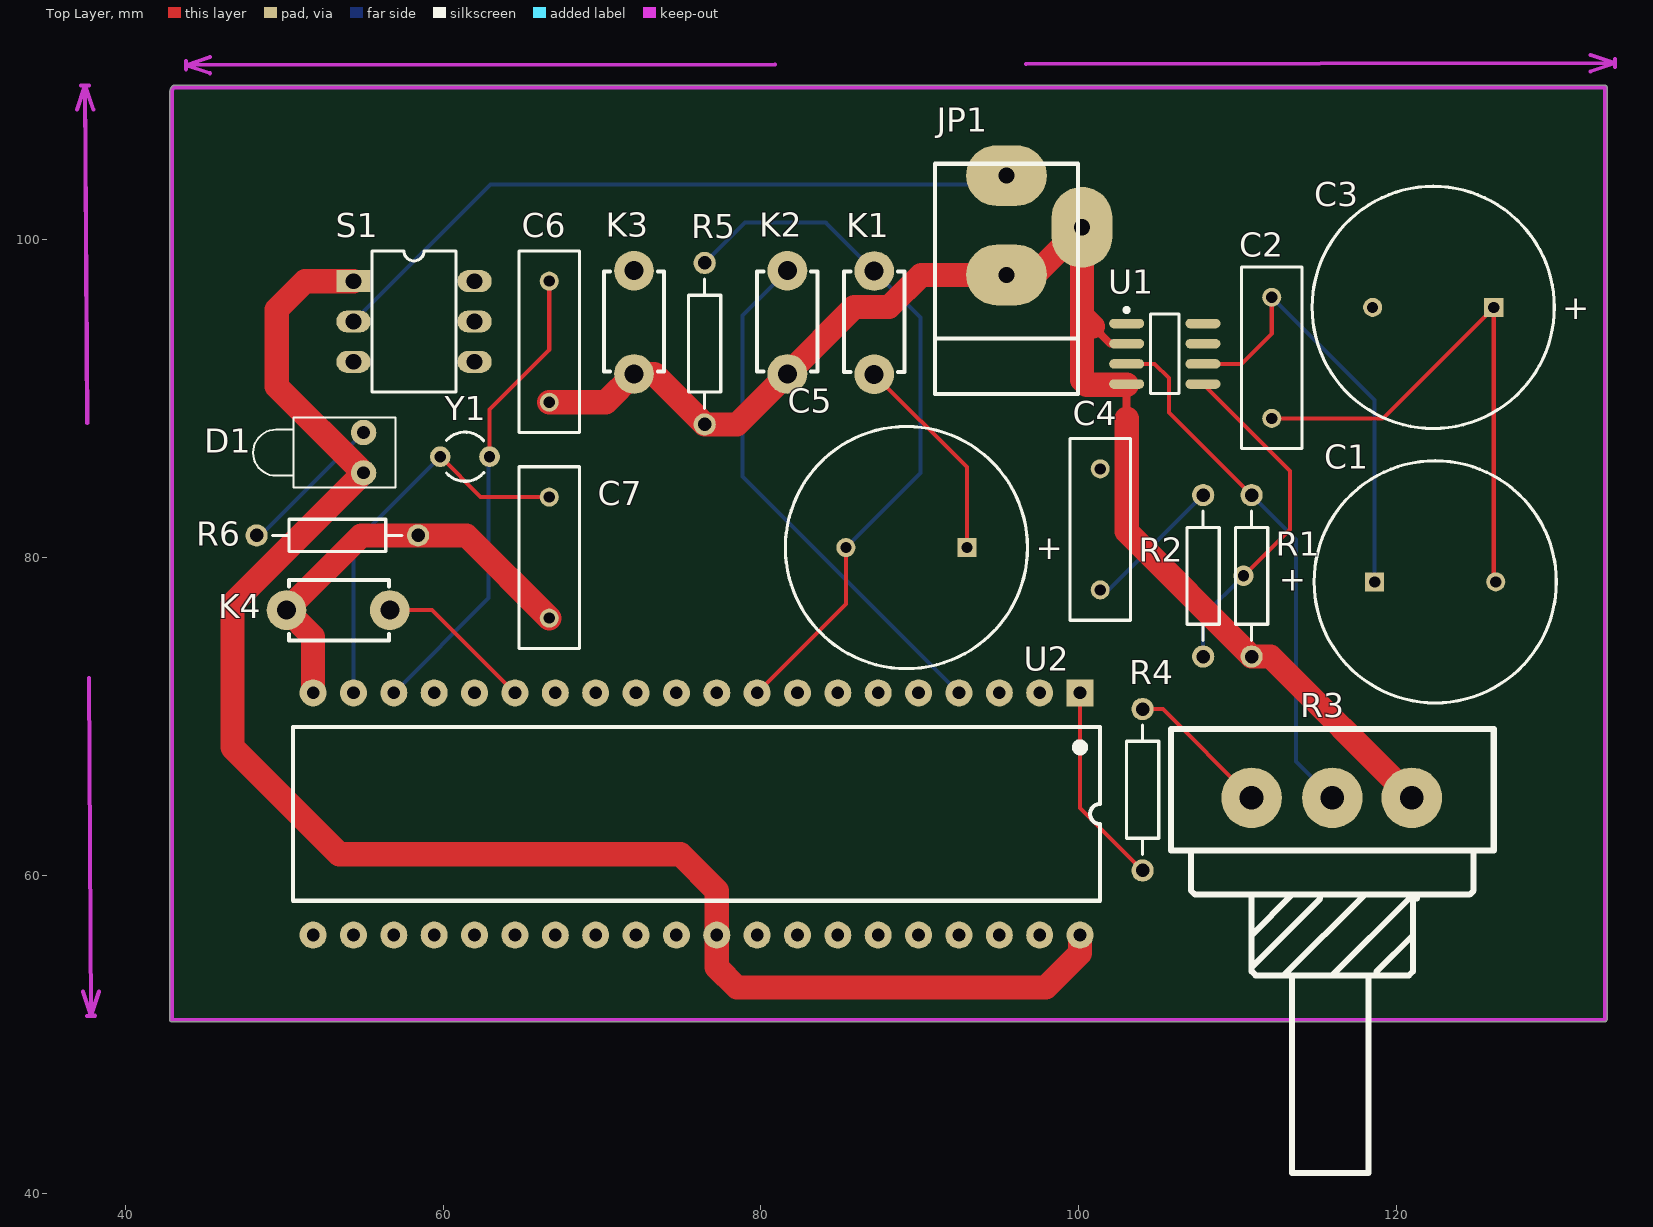
[diagram p0: Top Layer view]
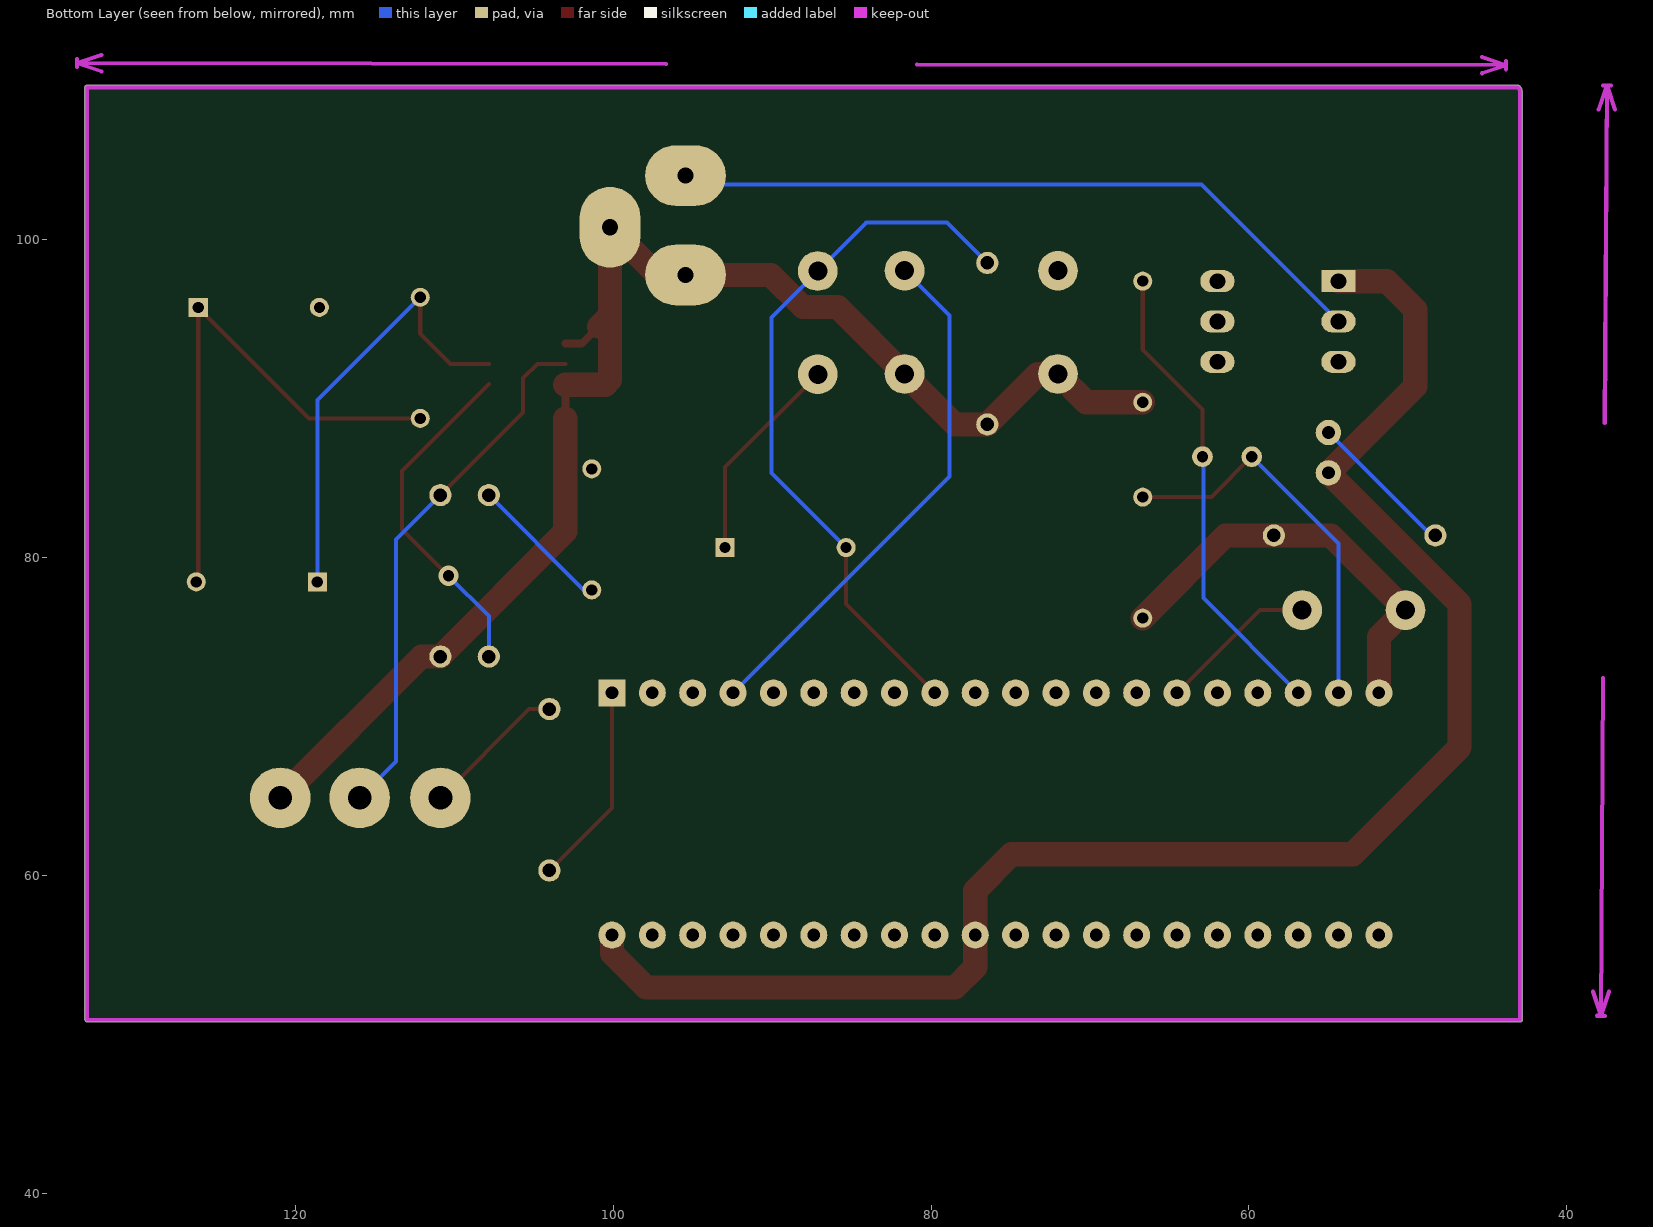
[diagram p1: Bottom Layer view, seen from below]
# Altium PCB MISC82808.PcbDoc
Units mm, origin at the board's own origin, x right, y up, seen from the top; angles counter-clockwise.
Board outline 90.45 x 58.93 mm, 2 copper layers (Top Layer, Bottom Layer); 23 components, 20 nets, 96 pads, 1 vias.
Unrouted connection lines stored in the file: 2.

## Layer stack, top to bottom (the 12.6 mil dielectric is the usual default, probably not edited)
Top Solder: solder mask 0.0102, Solder Resist, Dk 3.5
Top Layer: signal copper 0.0356
Dielectric 1: dielectric 0.32, FR-4, Dk 4.8
Bottom Layer: signal copper 0.0356
Bottom Solder: solder mask 0.0102, Solder Resist, Dk 3.5

## Board outline
42.926,50.8 cw(c42.926,50.927) 42.799,50.927 42.799,109.294 cw(c43.36,109.294) 42.963,109.691 cw(c43.053,109.601) 43.053,109.728 133.118,109.728 cw(c133.118,109.601) 133.245,109.601 133.245,50.98 cw(c133.043,50.98) 133.186,50.837 cw(c133.096,50.927) 133.096,50.8

## Design rules (kind name [scope] priority, off if disabled: settings)
Clearance [All] p1: gap=0.254
PolygonConnect [All] p1: connectstyle=Relief reliefconductorwidth=0.254 reliefentries=4 polygonreliefangle="90 Angle" airgapwidth=0.254
RoutingVias [All] p1: holewidth=0.711 width=1.27 viastyle="Through Hole" minholewidth=0.711 minwidth=1.27 maxholewidth=0.711 maxwidth=1.27
SolderMaskExpansion [All] p1: expansion=0.102
Width [All] p1: maxlimit=254 minlimit=0.254 preferedwidth=0.254 toplayer_maxwidth=25.4 minimp=50.000000 maximp=50.000000 favimp=50.000000
30 further rules are at their usual default settings.

## Classes and differential pairs
component class ZBW172: B1 C1 C3 C4 C5 C6 C7 D1 JP1 K1 K2 K3 K4 R3 R4 R5 R6 S1 U1 U2 Y1

## Components (designator, comment, footprint, x,y, rotation, side; value= is the part's Value field where it differs from the comment)
C1 "Cap Pol1" RB7.6-15 122.428,78.486 r180 top
C2 "Cap" RAD-0.3 112.141,92.583 r270 top
C3 "Cap Pol1" RB7.6-15 122.301,95.758 r0 top
C4 "Cap" RAD-0.3 101.346,81.788 r90 top
C5 "Cap Pol1" RB7.6-15 89.154,80.645 r0 top
C6 "Cap" RAD-0.3 66.675,93.599 r90 top
C7 "Cap" RAD-0.3 66.675,80.01 r90 top
D1 "LED1" LED-1 54.991,86.614 r180 top
JP1 "DC 5V" "DC POWER JACK1" 99.949,90.297 r90 top
K1 "KEY" DIP-3X6X4.3 87.122,91.544 r90 top
K2 "KEY" DIP-3X6X4.3 81.661,91.567 r90 top
K3 "KEY" DIP-3X6X4.3 72.009,91.567 r90 top
K4 "KEY" DIP-3X6X4.3 50.142,76.708 r0 top
R1 "Res2" AXIAL-0.4 110.871,78.867 r90 top
R2 "Res2" AXIAL-0.4 107.823,78.867 r90 top
R3 "Potentiometer" 滑动变阻器 115.951,55.245 r0 top
R4 "Res2" AXIAL-0.4 104.013,65.405 r90 top
R5 "Res2" AXIAL-0.4 76.454,93.472 r90 top
R6 "Res2" AXIAL-0.4 53.34,81.407 r0 top
S1 "SW3-DIP6" DIP-Switch3 54.356,97.409 r0 top
U1 "LM386" M08A_N 105.41,92.837 r0 top
U2 "STC89C51" DIP40 75.946,63.881 r270 top
Y1 "XTAL" R38 61.367,86.36 r90 top

## Footprints (in the part's own frame and the unit in brackets; to place one, negate y for a bottom-side part, rotate by r counter-clockwise, add the part's x,y. Pads: shape width x height; smd on the part's side, far side on the other; paste and mask are expansions set on the pad)
AXIAL-0.4 [mm] "Axial Device, Thru-Hole; 2 Leads; 0.4 in Pin Spacing"
  round 1.4 hole 0.85: 1(-5.08,0) 2(5.08,0)
  silkscreen extent -4.06,-1.02 4.06,1.02
"DC POWER JACK1" [mm] "ª½¬y¹q·½´¡®y"
  oval 3.81x5.08 hole 1.016: 1(13.75,4.5) 2(7.5,4.5)
  oval 5.08x3.81 hole 1.016: 3(10.5,-0.25)
  silkscreen extent 0,0 14.5,9
DIP40 [mm]
  rect 1.7x1.7 hole 0.8: 1(-7.62,24.13)
  round 1.7 hole 0.8: 2(-7.62,21.59) 3(-7.62,19.05) 4(-7.62,16.51) 5(-7.62,13.97) 6(-7.62,11.43) 7(-7.62,8.89) 8(-7.62,6.35) 9(-7.62,3.81) 10(-7.62,1.27) 11(-7.62,-1.27) 12(-7.62,-3.81) 13(-7.62,-6.35) 14(-7.62,-8.89) 15(-7.62,-11.43) 16(-7.62,-13.97) 17(-7.62,-16.51) 18(-7.62,-19.05) 19(-7.62,-21.59) 20(-7.62,-24.13) 21(7.62,-24.13) 22(7.62,-21.59) 23(7.62,-19.05) 24(7.62,-16.51) 25(7.62,-13.97) 26(7.62,-11.43) 27(7.62,-8.89) 28(7.62,-6.35) 29(7.62,-3.81) 30(7.62,-1.27) 31(7.62,1.27) 32(7.62,3.81) 33(7.62,6.35) 34(7.62,8.89) 35(7.62,11.43) 36(7.62,13.97) 37(7.62,16.51) 38(7.62,19.05) 39(7.62,21.59) 40(7.62,24.13)
  silkscreen extent -5.46,-25.4 5.46,25.4, body extent -7.91,-26.19 7.65,26.16, height 4.7
DIP-3X6X4.3 [mm]
  round 2.5 hole 1.2: 1(0,0) 3(6.5,0)
  silkscreen extent 0.16,-1.9 6.46,1.9, body extent -0.64,-1.75 7.19,1.75, height 4.31
DIP-Switch3 [mil]
  rect 85x55 hole 39 paste+0 mask+4: 1(0,0)
  oval 85x55 hole 39 paste+0 mask+4: 2(0,-100) 3(0,-200) 4(300,-200) 5(300,-100) 6(300,0)
  silkscreen extent 46,-275 254,75, body extent -55,-271 359,67, height 153
LED-1 [mm] "LED; 2 Leads"
  round 1.6 hole 0.8: 1(0,1.27) 2(0,-1.27)
  silkscreen extent -2,-2.2 6.95,2.2
M08A_N [mm] "SOIC, 8-Leads, Body 4.9x3.9mm, Pitch 1.27mm, IPC Medium Density"
  oval 2.2x0.6 smd: 1(-2.4,1.905) 2(-2.4,0.635) 3(-2.4,-0.635) 4(-2.4,-1.905) 5(2.4,-1.905) 6(2.4,-0.635) 7(2.4,0.635) 8(2.4,1.905)
  silkscreen extent -2.52,-2.5 0.9,2.88, body extent -2,-2.5 2,2.5, height 1.75
R38 [mm] "Crystal, Thru-Hole; 2 Leads; Body 3.1 x 8.2 mm (Dia.xH)"
  round 1.3 hole 0.7: 1(0,1.55) 2(0,-1.55)
  silkscreen extent -1.55,-1.19 1.55,1.17
RAD-0.3 [mm] "Radial Cap, Thru-Hole; 2 Leads; 0.3 in Pin Spacing"
  round 1.2 hole 0.7: 1(-3.81,0) 2(3.81,0)
  silkscreen extent -5.71,-1.91 5.71,1.91
RB7.6-15 [mm] "Polarized Capacitor (Radial); 2 Leads"
  rect 1.2x1.2 hole 0.7: 1(3.81,0)
  round 1.2 hole 0.7: 2(-3.81,0)
  silkscreen extent -7.62,-7.62 7.62,7.62
滑动变阻器 [mil]
  round 150 hole 59.06 paste+0 mask+4: 1(-200,380) 3(196.85,380)
  round 150 hole 59.05 paste+4 mask+4: 2(0,380)
  silkscreen extent -400,-550 400,550

## Part data
C1 C3 C5: "Polarized Capacitor (Radial)"
C2 C4 C6 C7: "Capacitor"
D1: "Typical RED GaAs LED"
JP1: library part "DC POWER JACK1", "DC power jack"
R1 R2 R4 R5 R6: "Resistor"
R3: library part 滑动变阻器
U1: library part LM386M-1, "Low Voltage Audio Power Amplifier, 8-pin Narrow SOIC"
Y1: "Crystal Oscillator"

## Via types
v1: diameter 1.27, hole 0.711, Top Layer to Bottom Layer, 1 vias

## Nets (pads, with @x,y where several pads share a name; then routed paths per layer and width w, separated by ;. In a path a pad name is that pad's centre, name@x,y a point inside that pad or via, vN(x,y) a via of type N, cw(c..) or ccw(c..) an arc to the next point about the centre after c; other vN are vias at no path point)
GND: C6.1 C7.1 JP1.2 JP1.3 K2.1 K3.1 K4.1 R1.1 R3.3 R5.1 R6.2 U1.2 U1.4 U2.20 | length 117.5
  Top Layer w0.508: 100.894,94.559 101.981,93.472 U1.2 ; 103.01,88.76 103.01,90.886 U1.4
  Top Layer w1.524: U2.20 51.816,75.034 K4.1 54.841,81.407 R6.2 61.468,81.407 C7.1 ; C6.1 70.231,89.789 K3.1 73.279,91.567 R5.1 78.486,88.392 K2.1 85.872,95.778 88.061,95.778 90.08,97.797 JP1.2 97.199,97.797 JP1.3 100.199,95.254 ; 100.894,94.559 100.199,95.254 ; 103.01,88.76 103.01,81.648 R1.1 112.061,73.787 R3.3 ; U1.4@103.01,90.886 100.495,90.886 100.199,91.182 100.199,95.254
NetB1_1: C4.2
NetB1_2: C3.2
NetC1_1: C1.1 C2.1 U1.6 | length 28
  Top Layer w0.254: U1.6 110.236,92.202 112.141,94.107 C2.1
  Bottom Layer w0.254: C2.1 118.618,89.916 C1.1
NetC1_2: C1.2 C2.2 C3.1 | length 34.2
  Top Layer w0.254: C2.2 119.126,88.773 C3.1 126.111,78.613 C1.2
NetC4_1: C4.1 R2.2 | length 8.9
  Bottom Layer w0.254: C4.1 101.854,77.978 R2.2
NetC5_1: C5.1 K1.1 | length 13.3
  Top Layer w0.254: K1.1 92.964,85.702 C5.1
NetC5_2: C5.2 K1.3 R5.2 U2.9 | length 45
  Top Layer w0.254: U2.9 85.344,77.089 C5.2
  Bottom Layer w0.254: R5.2 78.994,101.092 84.074,101.092 K1.3 90.043,95.123 90.043,85.344 C5.2
NetC6_2: C6.2 U2.18 Y1.2 | length 30
  Top Layer w0.254: Y1.2 62.917,89.333 66.675,93.091 C6.2
  Bottom Layer w0.254: U2.18 62.865,77.47 62.865,86.308 Y1.2
NetC7_2: C7.2 U2.19 Y1.1 | length 25
  Top Layer w0.254: Y1.1 62.357,83.82 C7.2
  Bottom Layer w0.254: U2.19 54.356,80.899 Y1.1
NetD1_2: D1.2 R6.1 | length 9.4
  Bottom Layer w0.254: R6.1 48.514,81.407 D1.2
NetJP1_1: JP1.1 S1.2 | length 44.9
  Bottom Layer w0.254: S1.2 62.992,103.505 94.907,103.505 JP1.1
NetR1_2: R1.2 R3.2 U1.3 | length 33.7
  Top Layer w0.254: U1.3 104.775,92.202 105.664,91.313 105.664,89.154 R1.2
  Bottom Layer w0.254: R1.2 113.665,81.153 113.665,67.183 R3.2
NetR2_1: R2.1 U1.5 | length 21.7
  Top Layer w0.254: U1.5 113.284,85.458 113.284,81.788 v1(110.363,78.867)
  Bottom Layer w0.254: R2.1 107.823,76.327 v1(110.363,78.867)
NetR3_1: R3.1 R4.2 | length 9.2
  Top Layer w0.254: R4.2 105.283,70.485 R3.1
NetR4_1: R4.1 U2.1 | length 12.8
  Top Layer w0.254: U2.1 100.076,64.262 R4.1
P1.3: K2.3 U2.4 | length 33.4
  Bottom Layer w0.254: K2.3 78.844,95.25 78.844,85.113 U2.4
P3.2: K3.3 U2.12
P3.5: K4.3 U2.15 | length 10
  Top Layer w0.254: K4.3 59.309,76.708 U2.15
VCC: D1.1 S1.1 U2.31 U2.40 | length 103.3
  Top Layer w1.524: S1.1 51.308,97.409 49.53,95.631 49.53,90.777 54.963,85.344 D1.1 46.736,77.089 46.736,68.072 53.467,61.341 74.93,61.341 77.216,59.055 U2.31 77.216,54.229 78.486,52.959 97.917,52.959 100.076,55.118 U2.40
pads on no net: S1.3 S1.4 S1.5 S1.6 U1.1 U1.7 U1.8 U2.2 U2.3 U2.5 U2.6 U2.7 U2.8 U2.10 U2.11 U2.13 U2.14 U2.16 U2.17 U2.21 U2.22 U2.23 U2.24 U2.25 U2.26 U2.27 U2.28 U2.29 U2.30 U2.32 U2.33 U2.34 U2.35 U2.36 U2.37 U2.38 U2.39

## Keep-outs
Keep-Out Layer:
  lines w0.254: 36.967,108.201 37.465,109.728 ; 37.211,109.726 37.719,109.73 ; 37.328,52.702 37.846,51.181 ; 37.592,51.179 38.1,51.183 ; 37.603,88.478 37.465,109.728 ; 37.708,72.431 37.846,51.181 ; 37.983,108.207 37.465,109.728 ; 38.344,52.708 37.846,51.181 ; 43.815,110.744 43.815,111.252 ; 44.196,109.601 43.053,109.601 ; 45.338,111.508 43.815,110.998 ; 45.34,110.492 43.815,110.998 ; 80.876,111.05 43.815,110.998 ; 96.67,111.073 133.731,111.125 ; 132.206,111.631 133.731,111.125 ; 132.208,110.615 133.731,111.125 ; 133.731,110.871 133.731,111.379 ; 43.053,109.601 ccw(c43.36,109.294) 42.926,109.294 42.926,51.181 42.926,50.927 133.096,50.927 ccw(c133.043,50.98) 133.118,50.98 133.118,109.601 43.053,109.601
  text "89.916 (mm)" at 81.131,110.137 h1.52 r0.08
  text "58.548 (mm)" at 36.691,88.218 h1.52 r270.37